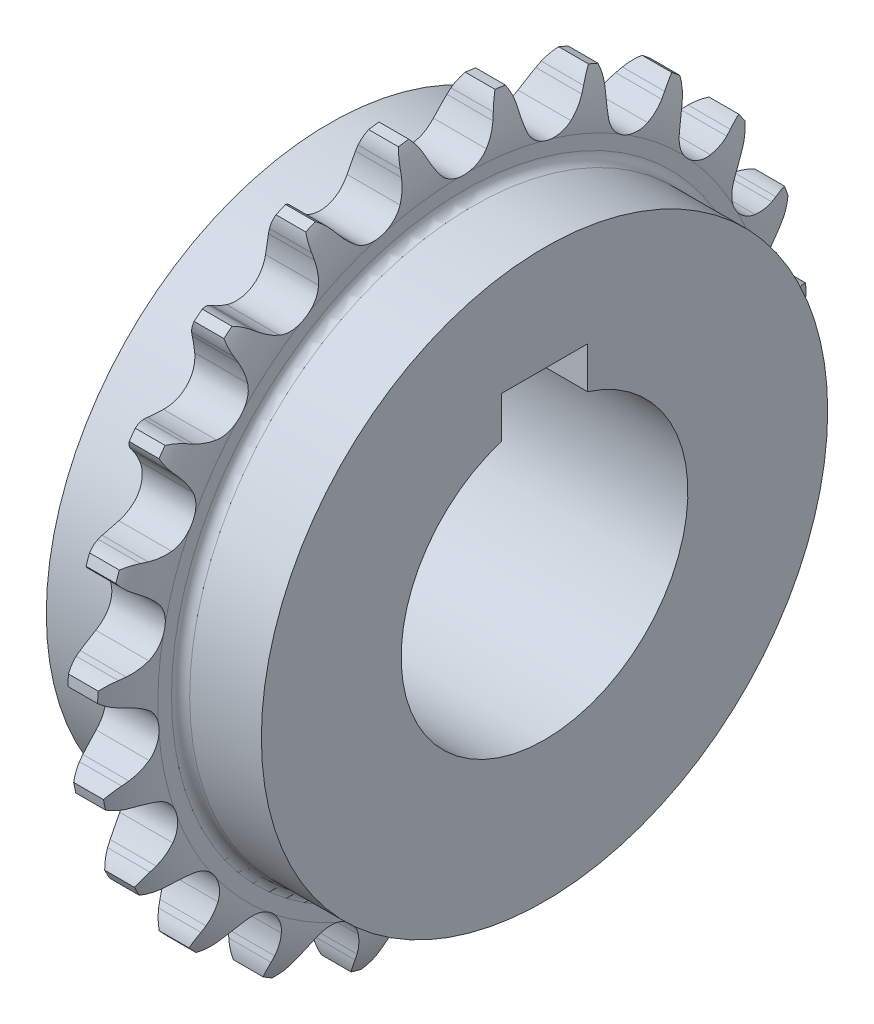
from build123d import *

# Parameters (mm, degrees)
EXTRUDECUTONE_DEPTH      = 5.315766473
PATTERNONE_COUNT         = 23
SKETCH_1_2_R             = 39.5
EXTRUDE_1_DEPTH          = 15
CUT_EXTRUDE_B_DEPTH      = 72.543477978
CUT_EXTRUDE_B_DEPTH_BACK = 72.543477978


with BuildPart() as part:
    # Sketch 1 → Revolve 2 (revolve)
    with BuildSketch(Plane.XY, mode=Mode.PRIVATE) as revolve_2_sk:
        with BuildLine():
            Line((-5.315766473, 0), (-5.315766473, 39.5))
            Line((-5.315766473, 39.5), (-4.998363178, 39.5))
            ThreePointArc((-4.998363178, 39.5), (-4.10061109, 39.87186109), (-3.72875, 40.769613178))
            Line((-3.72875, 40.769613178), (-3.72875, 42.674032945))
            ThreePointArc((-3.72875, 42.674032945), (-3.384453661, 46.203405438), (-2.07775, 49.5))
            Line((-2.07775, 49.5), (2.07775, 49.5))
            ThreePointArc((2.07775, 49.5), (3.384453661, 46.203405438), (3.72875, 42.674032945))
            Line((3.72875, 42.674032945), (3.72875, 40.769613178))
            ThreePointArc((3.72875, 40.769613178), (4.10061109, 39.87186109), (4.998363178, 39.5))
            Line((4.998363178, 39.5), (5.315766473, 39.5))
            Line((5.315766473, 39.5), (5.315766473, 0))
            Line((5.315766473, 0), (-5.315766473, 0))
        make_face()
    revolve(revolve_2_sk.sketch.rotate(Axis((-4, 0, 0), (1, 0, 0)), 90), axis=Axis((-4, 0, 0), (1, 0, 0)))

    # 草图2 → ExtrudeCutOne (cut, symmetric)
    with BuildSketch(Plane(origin=(0, 0, 0), x_dir=(0, 0, -1), z_dir=(1, 0, 0))):
        with BuildLine():
            Line((4.588692581, 46.610285416), (4.899653292, 47.378261808))
            ThreePointArc((4.899653292, 47.378261808), (5.378614734, 48.306828579), (6.018529669, 49.132751812))
            ThreePointArc((6.018529669, 49.132751812), (0, 49.5), (-6.018529669, 49.132751812))
            ThreePointArc((-6.018529669, 49.132751812), (-5.378614734, 48.306828579), (-4.899653292, 47.378261808))
            Line((-4.899653292, 47.378261808), (-4.588692581, 46.610285416))
            ThreePointArc((-4.588692581, 46.610285416), (-3.973376288, 45.345046883), (-3.192395607, 44.174785433))
            ThreePointArc((-3.192395607, 44.174785433), (0, 42.604232945), (3.192395607, 44.174785433))
            ThreePointArc((3.192395607, 44.174785433), (3.973376288, 45.345046883), (4.588692581, 46.610285416))
        make_face()
    extrudecutone = extrude(amount=EXTRUDECUTONE_DEPTH, both=True, mode=Mode.SUBTRACT)

    # PatternOne: ExtrudeCutOne ×23 about axis
    patternone_axis = Axis((0, 0, 0), (1, 0, 0))
    for i in range(1, PATTERNONE_COUNT):
        add(extrudecutone.rotate(patternone_axis, i * 360 / PATTERNONE_COUNT), mode=Mode.SUBTRACT)

    # Sketch 1 2 → 凸台-拉伸1 (add, symmetric)
    with BuildSketch(Plane(origin=(0, 0, 0), x_dir=(0, 0, -1), z_dir=(1, 0, 0))):
        with Locations(Location((0, 0, 0), (0, 0, 180))):
            Circle(SKETCH_1_2_R)
    extrude(amount=EXTRUDE_1_DEPTH, both=True)

    # 草图Key → 切除-拉伸B (cut, two sides: drawn at the far end of the back side and taken through both)
    with BuildSketch(Plane(origin=(0, 0, 0), x_dir=(0, 0, -1), z_dir=(1, 0, 0)).offset(-CUT_EXTRUDE_B_DEPTH_BACK)):
        with BuildLine():
            Line((-6, 19.078784028), (-6, 24.860608081))
            Line((-6, 24.860608081), (6, 24.860608081))
            Line((6, 24.860608081), (6, 19.078784028))
            ThreePointArc((6, 19.078784028), (0, -20), (-6, 19.078784028))
        make_face()
    extrude(amount=CUT_EXTRUDE_B_DEPTH + CUT_EXTRUDE_B_DEPTH_BACK, mode=Mode.SUBTRACT)


solid = part.part
